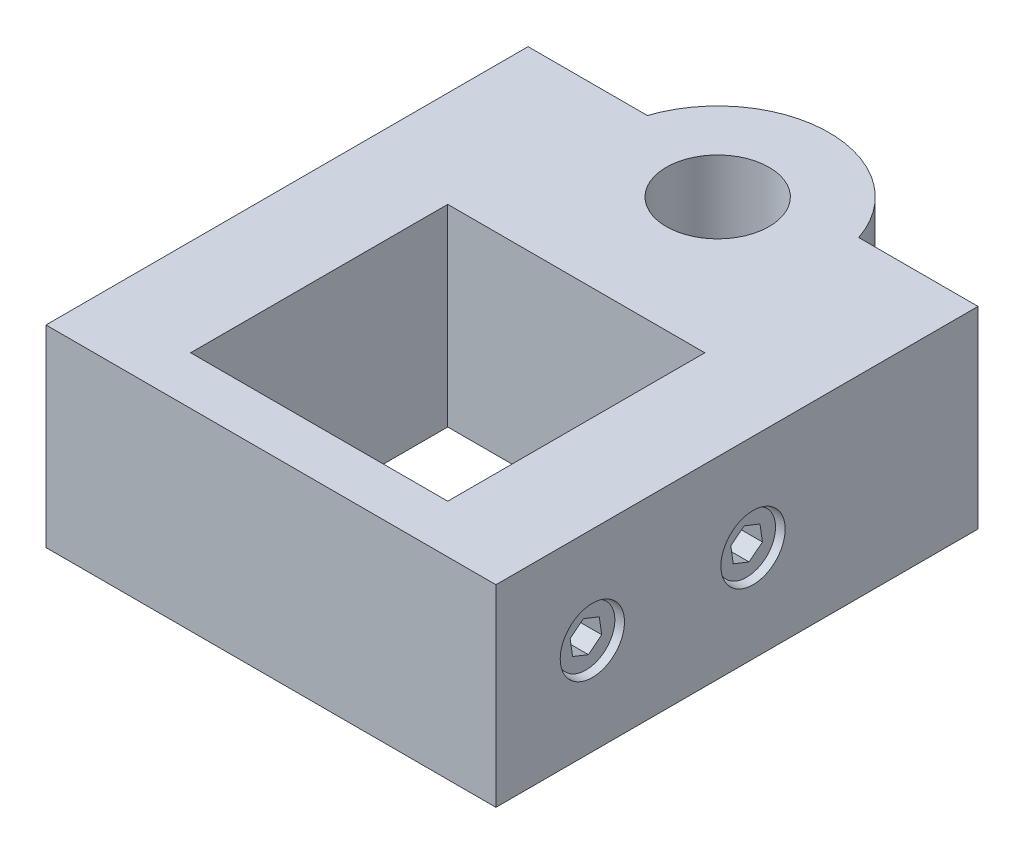
from build123d import *

# Parameters (mm, degrees)
SKETCH1_W           = 70
SKETCH1_H           = 55
SKETCH1_W_2         = 40
SKETCH1_H_2         = 40
BOSS_EXTRUDE1_DEPTH = 30
SKETCH2_W           = 70
SKETCH2_H           = 20
BOSS_EXTRUDE2_DEPTH = 30
SKETCH3_R           = 8
CUT_EXTRUDE1_DEPTH  = 30
SKETCH4_R           = 17.338439929
SKETCH4_R_2         = 8
BOSS_EXTRUDE3_DEPTH = 30
SKETCH5_R           = 5
CUT_EXTRUDE2_DEPTH  = 6
SKETCH6_R           = 4.5
BOSS_EXTRUDE4_DEPTH = 5


with BuildPart() as part:
    # Sketch1 → Boss-Extrude1 (new body)
    with BuildSketch(Plane(origin=(0, 0, 0), x_dir=(1, 0, 0), z_dir=(0, 1, 0))):
        Rectangle(SKETCH1_W, SKETCH1_H)
        Rectangle(SKETCH1_W_2, SKETCH1_H_2, mode=Mode.SUBTRACT)
    extrude(amount=BOSS_EXTRUDE1_DEPTH)

    # Sketch2 → Boss-Extrude2 (add)
    with BuildSketch(Plane(origin=(0, 30, 0), x_dir=(1, 0, 0), z_dir=(0, 1, 0))):
        with Locations((0, 37.5)):
            Rectangle(SKETCH2_W, SKETCH2_H)
    extrude(amount=-BOSS_EXTRUDE2_DEPTH)

    # Sketch3 → Cut-Extrude1 (cut)
    with BuildSketch(Plane.XZ):
        with Locations((0, -42)):
            Circle(SKETCH3_R)
    extrude(amount=-CUT_EXTRUDE1_DEPTH, mode=Mode.SUBTRACT)

    # Sketch4 → Boss-Extrude3 (add)
    with BuildSketch(Plane.XZ):
        with Locations((0, -42)):
            Circle(SKETCH4_R)
        with Locations(Location((0, -42, 0), (0, 0, 270))):
            Circle(SKETCH4_R_2, mode=Mode.SUBTRACT)
    extrude(amount=-BOSS_EXTRUDE3_DEPTH)

    # Sketch5 → Cut-Extrude2 (cut)
    with BuildSketch(Plane.ZY.offset(35)):
        with Locations((12.5, 15)):
            Circle(SKETCH5_R)
        with Locations((-12.5, 15)):
            Circle(SKETCH5_R)
    cut_extrude2 = extrude(amount=-CUT_EXTRUDE2_DEPTH, mode=Mode.SUBTRACT)

    # Sketch6 → Boss-Extrude4 (add)
    # profile 1 of 2: a face of its own
    with BuildSketch(Plane.ZY.offset(29)):
        with Locations((-12.5, 15)):
            Circle(SKETCH6_R)
        Polygon((-10.422763648, 13.355760931), (-10.03742902, 15.976819916), (-12.114665372, 17.621058985), (-14.577236352, 16.644239069), (-14.96257098, 14.023180084), (-12.885334628, 12.378941015), align=None, mode=Mode.SUBTRACT)
    # profile 2 of 2: a face of its own
    with BuildSketch(Plane.ZY.offset(29)):
        with Locations((12.5, 15)):
            Circle(SKETCH6_R)
        Polygon((14.569670203, 13.355760931), (14.958787905, 15.970267439), (12.889117702, 17.614506508), (10.430329797, 16.644239069), (10.041212095, 14.029732561), (12.110882298, 12.385493492), align=None, mode=Mode.SUBTRACT)
    boss_extrude4 = extrude(amount=BOSS_EXTRUDE4_DEPTH)

    # Mirror1: Cut-Extrude2, Boss-Extrude4 across plane
    add(cut_extrude2.mirror(Plane(origin=(0, 0, 0), x_dir=(0, 0, 1), z_dir=(1, 0, 0))), mode=Mode.SUBTRACT)
    add(boss_extrude4.mirror(Plane(origin=(0, 0, 0), x_dir=(0, 0, 1), z_dir=(1, 0, 0))))


solid = part.part
